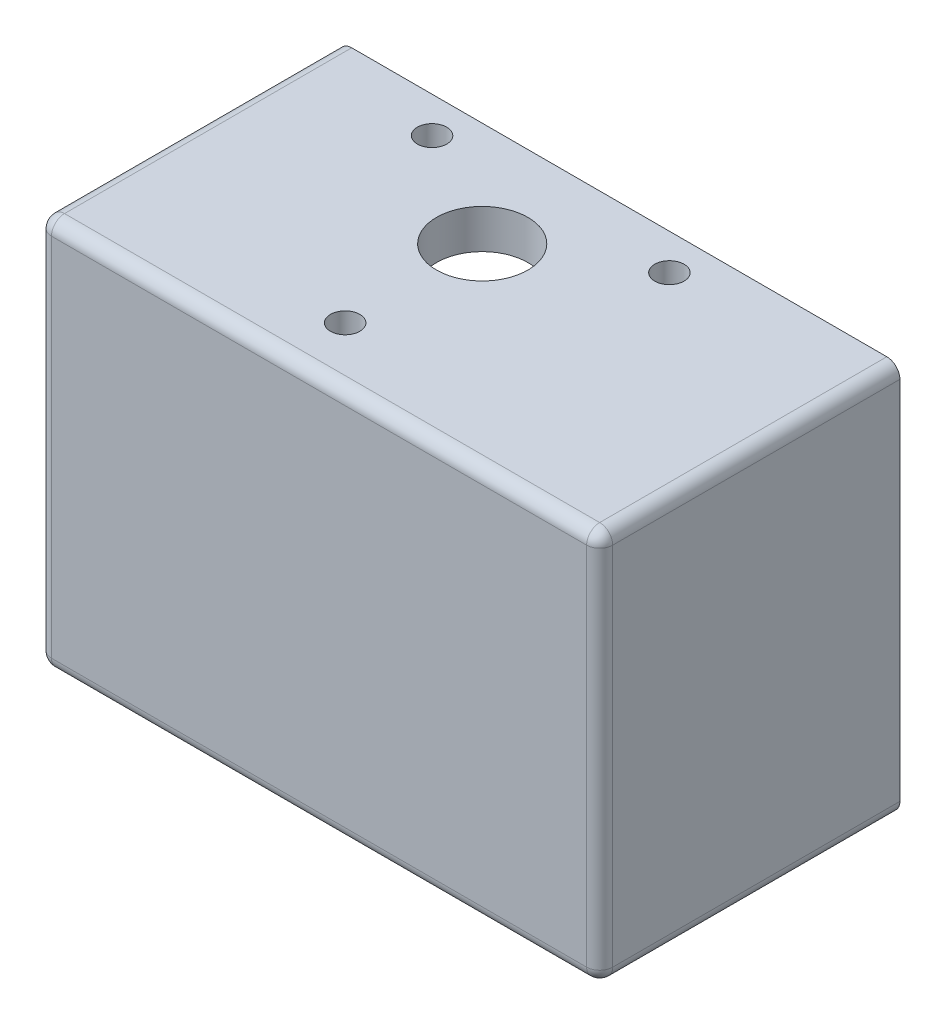
SolidWorks part; units mm, degrees
material "6061 合金"
ref_plane "前视基准面" through (0, 0, 0) normal (0, 0, 1) x (1, 0, 0)
ref_plane "上视基准面" through (0, 0, 0) normal (0, 1, 0) x (1, 0, 0)
ref_plane "右视基准面" through (0, 0, 0) normal (1, 0, 0) x (0, 0, -1)
sketch "草图1" plane through (0, 0, 0) normal (0, 0, 1) x (1, 0, 0)
  line L1 (-43, 30) -> (43, 30)
  line L2 (-43, 30) -> (-43, -30)
  line L3 (-43, -30) -> (43, -30)
  line L4 (43, 30) -> (43, -30)
  line L5 (-43, 30) -> (43, -30) construction
  line L6 (-43, -30) -> (43, 30) construction
  point P0 (0, 0)
  dimension "D1" = 60
  dimension "D2" = 86
extrude "凸台-拉伸1" add sketch "草图1" along normal blind 46
sketch "草图2" plane through (0, 0, 0) normal (0, 0, -1) x (-1, 0, 0)
  line L14 (37, -24) -> (37, 24)
  line L15 (-37, -24) -> (37, -24)
  line L16 (-37, 24) -> (-37, -24)
  line L17 (37, 24) -> (-37, 24)
  line L18 (37, -24) -> (37, 24)
  line L19 (-37, -24) -> (37, -24)
  line L20 (-37, 24) -> (-37, -24)
  line L21 (37, 24) -> (-37, 24)
  dimension "D1" = 6
extrude "切除-拉伸1" cut sketch "草图2" against normal blind 41
fillet "圆角1" radius 5 4 edges at (37, -24, 20.5) (-37, -24, 20.5) (-37, 24, 20.5) (37, 24, 20.5)
sketch "草图3" plane through (0, -30, 0) normal (0, -1, 0) x (1, 0, 0)
  line L1 (27, 46) -> (27, 0) construction
  line L2 (-5, 46) -> (-5, 0)
  line L3 (-5, 46) -> (-5, 0) construction
  line L4 (-27, 46) -> (-27, 0) construction
  line L6 (-49.7845, 9) -> (51.8038, 9) construction
  line L7 (-43, 16) -> (43, 16)
  line L8 (-43, 16) -> (43, 16) construction
  line L9 (-43, 31) -> (43, 31) construction
  line L10 (25, 9) -> (29, 9) construction
  line L11 (25, 11.75) -> (29, 11.75)
  line L12 (25, 6.25) -> (29, 6.25)
  line L13 (25, 31) -> (29, 31) construction
  line L14 (25, 33.75) -> (29, 33.75)
  line L15 (25, 28.25) -> (29, 28.25)
  line L16 (-29, 31) -> (-25, 31) construction
  line L17 (-29, 33.75) -> (-25, 33.75)
  line L18 (-29, 28.25) -> (-25, 28.25)
  line L19 (-29, 9) -> (-25, 9) construction
  line L20 (-29, 11.75) -> (-25, 11.75)
  line L21 (-29, 6.25) -> (-25, 6.25)
  circle A0 centre (-5, 16) radius 7
  arc A1 (25, 11.75) -> (25, 6.25) centre (25, 9) ccw
  arc A2 (29, 6.25) -> (29, 11.75) centre (29, 9) ccw
  arc A3 (25, 33.75) -> (25, 28.25) centre (25, 31) ccw
  arc A4 (29, 28.25) -> (29, 33.75) centre (29, 31) ccw
  arc A5 (-29, 33.75) -> (-29, 28.25) centre (-29, 31) ccw
  arc A6 (-25, 28.25) -> (-25, 33.75) centre (-25, 31) ccw
  arc A7 (-29, 11.75) -> (-29, 6.25) centre (-29, 9) ccw
  arc A8 (-25, 6.25) -> (-25, 11.75) centre (-25, 9) ccw
  point P16 (27, 9)
  point P21 (27, 31)
  point P28 (-27, 31)
  point P35 (-27, 9)
  dimension "D5" = 14
  dimension "D11" = 2.75
  dimension "D12" = 2.75
  dimension "D13" = 2.75
  dimension "D14" = 2.75
  dimension "D7" = 4
  dimension "D8" = 4
  dimension "D9" = 4
  dimension "D10" = 4
  dimension "D1" = 38
  dimension "D2" = 32
  dimension "D3" = 22
  dimension "D4" = 16
  dimension "D6" = 15
extrude "切除-拉伸3" cut sketch "草图3" against normal blind 7
sketch "草图4" plane through (0, 30, 0) normal (0, 1, 0) x (1, 0, 0)
  line L0 (-5, 3.8488) -> (-5, -43.5235) construction
  line L1 (-32.9722, -16) -> (30.4152, -16) construction
  line L2 (-5, -16) -> (19.7279, -1.7233) construction
  line L3 (-5, -16) -> (-32.2726, -0.2542) construction
  circle A0 centre (-5, -16) radius 7
  circle A1 centre (-5, -16) radius 21 construction
  circle A2 centre (13.1865, -5.5) radius 2.25
  circle A3 centre (-5, -37) radius 2.25
  circle A4 centre (-23.1865, -5.5) radius 2.25
  dimension "D1" = 42
  dimension "D4" = 4.5
  dimension "D5" = 4.5
  dimension "D6" = 4.5
  dimension "D2" = 120
  dimension "D3" = 120
extrude "切除-拉伸4" cut sketch "草图4" against normal blind 7
sketch "草图5" plane through (-43, 0, 0) normal (-1, 0, 0) x (0, 0, 1)
  line L1 (-20.6218, 0) -> (58.7237, 0) construction
  line L2 (16, 30) -> (16, -30)
  line L3 (16, 30) -> (16, -30) construction
  circle A0 centre (16, 0) radius 8.5
  dimension "D2" = 17
  dimension "D1" = 16
extrude "切除-拉伸5" cut sketch "草图5" against normal blind 7
sketch "草图6" plane through (-43, 0, 0) normal (-1, 0, 0) x (0, 0, 1)
  line L0 (-15.7614, 0) -> (50.4611, 0) construction
  line L1 (16, 19.2592) -> (16, -23.755) construction
  line L2 (16, 0) -> (5.5818, 18.0449) construction
  line L3 (16, 0) -> (4.552, -19.8284) construction
  circle A0 centre (16, 0) radius 13.5 construction
  dimension "D1" = 27
  dimension "D2" = 120
  dimension "D3" = 120
hole_wizard "M3 螺纹孔2" positions "3D草图2" profile "草图9" tap size "M3" standard "GB"
sketch3d "3D草图2"
  line L0 (-43, 0, -15.7614) -> (-43, 0, 50.4611) construction
  line L1 (-43, 0, 16) -> (-43, -19.8284, 4.552) construction
  line L2 (-43, 0, 16) -> (-43, 18.0449, 5.5818) construction
  circle A0 centre (-43, 0, 16) radius 13.5 construction
  point P0 (-43, 0, 29.5)
  point P6 (-56.5, 0, 16)
  point P7 (-43, -11.6913, 9.25)
  point P11 (-43, 11.6913, 9.25)
sketch "草图9" plane through (-43, 0, 29.5) normal (0, 1, 0) x (0, 0, 1)
  line L0 (0, 0) -> (0, 9.2511)
  line L1 (0, 9.2511) -> (1.25, 8.5)
  line L2 (1.25, 8.5) -> (1.25, 0)
  line L5 (1.25, 0) -> (0, 0)
  line L10 (0, 9.2511) -> (-1.25, 8.5) construction
  line L11 (0, -6.35) -> (0, 107.95) construction
  dimension "螺纹孔钻头直径" = 2.5
  dimension "螺纹孔钻头深度" = 8.5
  dimension "导头角度" = 118
cosmetic thread "孔螺蚊线4" parameters "D1"=6, "D2"=3
cosmetic thread "孔螺蚊线5" parameters "D1"=6, "D2"=3
cosmetic thread "孔螺蚊线6" parameters "D1"=6, "D2"=3
sketch "草图10" plane through (0, 0, 0) normal (0, 0, -1) x (-1, 0, 0)
  line L2 (-43, 25) -> (43, 25)
  line L3 (-43, 25) -> (43, 25) construction
  line L5 (43, -25) -> (-43, -25)
  line L6 (43, -25) -> (-43, -25) construction
  line L15 (-39.5, -30) -> (-39.5, 30)
  line L16 (-39.5, -30) -> (-39.5, 30) construction
  line L18 (39.5, 30) -> (39.5, -30)
  line L19 (39.5, 30) -> (39.5, -30) construction
  dimension "D1" = 5
  dimension "D2" = 5
  dimension "D3" = 3.5
  dimension "D4" = 3.5
hole_wizard "M3 螺纹孔3" positions "3D草图3" profile "草图11" tap size "M3" standard "GB"
sketch3d "3D草图3"
  line L0 (43, 25, 0) -> (-43, 25, 0) construction
  line L1 (39.5, -30, 0) -> (39.5, 30, 0) construction
  line L2 (-39.5, 30, 0) -> (-39.5, -30, 0) construction
  line L3 (-43, -25, 0) -> (43, -25, 0) construction
  point P0 (39.5, 25, 0)
  point P6 (-39.5, 25, 0)
  point P10 (-39.5, -25, 0)
  point P14 (39.5, -25, 0)
sketch "草图11" plane through (39.5, 25, 0) normal (1, 0, 0) x (0, 1, 0)
  line L0 (0, 0) -> (0, 9.2511)
  line L1 (0, 9.2511) -> (1.25, 8.5)
  line L2 (1.25, 8.5) -> (1.25, 0)
  line L5 (1.25, 0) -> (0, 0)
  line L10 (0, 9.2511) -> (-1.25, 8.5) construction
  line L11 (0, -6.35) -> (0, 107.95) construction
  dimension "螺纹孔钻头直径" = 2.5
  dimension "螺纹孔钻头深度" = 8.5
  dimension "导头角度" = 118
cosmetic thread "孔螺蚊线7" parameters "D1"=6, "D2"=3
cosmetic thread "孔螺蚊线8" parameters "D1"=6, "D2"=3
cosmetic thread "孔螺蚊线9" parameters "D1"=6, "D2"=3
cosmetic thread "孔螺蚊线10" parameters "D1"=6, "D2"=3
fillet "圆角2" radius 2 8 edges at (43, -30, 23) (43, 30, 23) (-43, -30, 23) (-43, 30, 23) (-43, 0, 46) (0, -30, 46) (43, 0, 46) (0, 30, 46)
